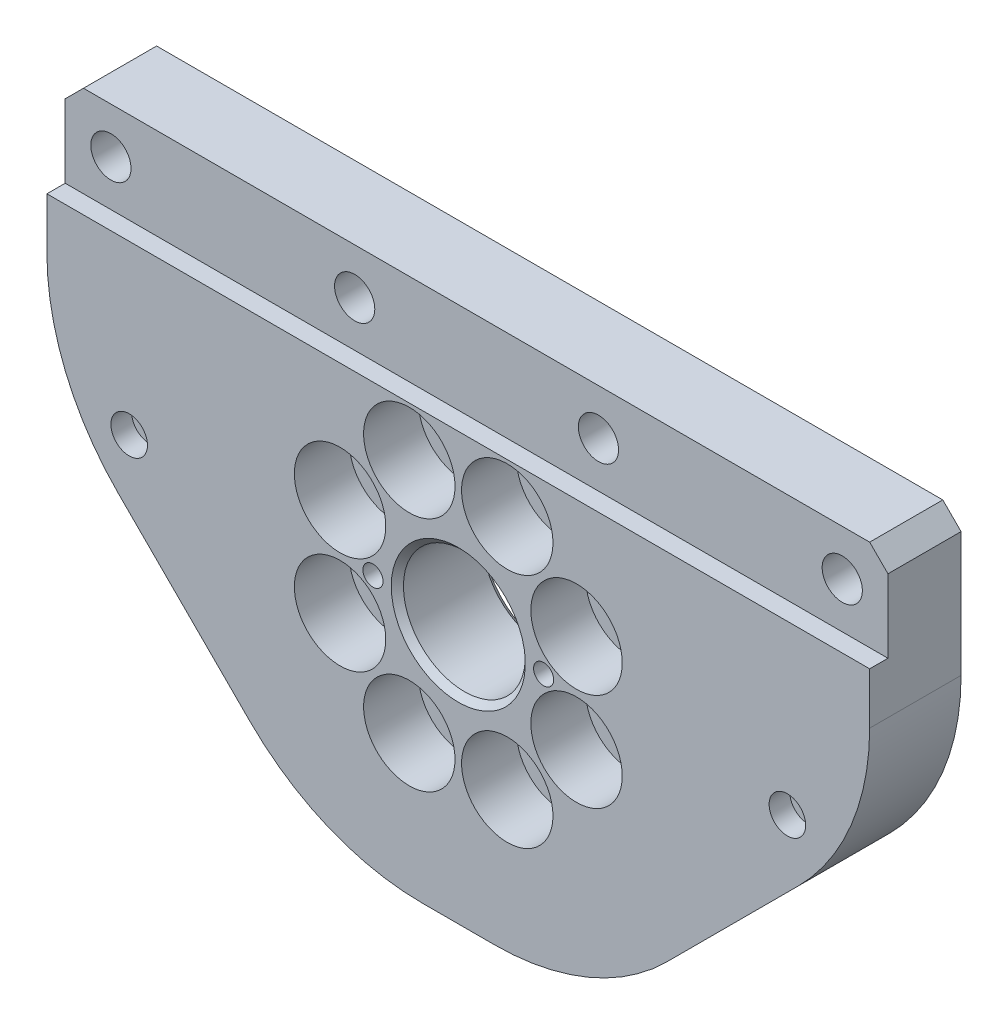
from build123d import *

# Parameters (mm, degrees)
SKETCH_1_R                  = 10
EXTRUDE_1_DEPTH             = 7.5
HOLE_WIZARD_2_D             = 9
HOLE_WIZARD_2_CBORE_D       = 15
HOLE_WIZARD_2_CBORE_DEPTH   = 9
CHAMFER_1_SIZE              = 1
PATTERN_CIRCULAR_1_COUNT    = 8
HOLE_WIZARD_2_2_D           = 3.4
HOLE_WIZARD_2_2_CBORE_D     = 6
HOLE_WIZARD_2_2_CBORE_DEPTH = 3.4
HOLE_WIZARD_8_0_8_1_D       = 8
HOLE_WIZARD_8_0_8_1_DEPTH   = 8
HOLE_WIZARD_8_0_8_1_TIP     = 2.403442476
HOLE_WIZARD_M4_1_D          = 3.3
SKETCH_10_W                 = 135
SKETCH_10_H                 = 15
CUT_EXTRUDE_1_DEPTH         = 3
HOLE_WIZARD_3_D             = 6.6
HOLE_WIZARD_3_CBORE_D       = 11
HOLE_WIZARD_3_CBORE_DEPTH   = 6.8
CHAMFER_2_SIZE              = 3


with BuildPart() as part:
    # 草图1 → 凸台-拉伸1 (new, symmetric)
    with BuildSketch(Plane.XY):
        with BuildLine():
            Line((-55.784271247, -9.215728753), (-34.215728753, -30.784271247))
            ThreePointArc((-34.215728753, -30.784271247), (-21.2387948, -39.4551813), (-5.931457505, -42.5))
            Line((-5.931457505, -42.5), (5.931457505, -42.5))
            ThreePointArc((5.931457505, -42.5), (21.2387948, -39.4551813), (34.215728753, -30.784271247))
            Line((34.215728753, -30.784271247), (55.784271247, -9.215728753))
            ThreePointArc((55.784271247, -9.215728753), (64.4551813, 3.7612052), (67.5, 19.068542495))
            Line((67.5, 19.068542495), (67.5, 42.5))
            Line((67.5, 42.5), (-67.5, 42.5))
            Line((-67.5, 42.5), (-67.5, 19.068542495))
            ThreePointArc((-67.5, 19.068542495), (-64.4551813, 3.7612052), (-55.784271247, -9.215728753))
        make_face()
        Circle(SKETCH_1_R, mode=Mode.SUBTRACT)
    extrude(amount=EXTRUDE_1_DEPTH, both=True)

    # Hole Wizard 2 (through all)
    with Locations(Plane.XY.offset(7.5)):
        with Locations((-8.03635208, 19.401470183)):
            hole_wizard_2 = CounterBoreHole(HOLE_WIZARD_2_D / 2, HOLE_WIZARD_2_CBORE_D / 2, HOLE_WIZARD_2_CBORE_DEPTH)

    # 倒角1
    chamfer_1_edges = [part.edges().sort_by_distance(p)[0] for p in [
        (-10, 0, -7.5),
        (-10, 0, 7.5),
    ]]
    chamfer(chamfer_1_edges, length=CHAMFER_1_SIZE)

    # 阵列(圆周)1: Hole Wizard 2 ×8 about axis
    pattern_circular_1_axis = Axis((0, 0, 0), (0, 0, 1))
    for i in range(1, PATTERN_CIRCULAR_1_COUNT):
        add(hole_wizard_2.rotate(pattern_circular_1_axis, i * 360 / PATTERN_CIRCULAR_1_COUNT), mode=Mode.SUBTRACT)

    # Hole Wizard 2 2 (through all)
    with Locations(Plane.XY.offset(7.5)):
        with Locations((-54, 0), (54, 0)):
            CounterBoreHole(HOLE_WIZARD_2_2_D / 2, HOLE_WIZARD_2_2_CBORE_D / 2, HOLE_WIZARD_2_2_CBORE_DEPTH)

    # Ø8.0 (8) 直径孔1
    with Locations(Plane(origin=(0, 0, -7.5), x_dir=(-1, 0, 0), z_dir=(0, 0, -1))):
        with Locations((-54, 0), (54, 0)):
            Hole(HOLE_WIZARD_8_0_8_1_D / 2, depth=HOLE_WIZARD_8_0_8_1_DEPTH)
            with Locations((0, 0, -(HOLE_WIZARD_8_0_8_1_DEPTH + HOLE_WIZARD_8_0_8_1_TIP / 2))):  # 118° drill point
                Cone(0, HOLE_WIZARD_8_0_8_1_D / 2, HOLE_WIZARD_8_0_8_1_TIP, mode=Mode.SUBTRACT)

    # M4 螺纹孔1 (through all)
    with Locations(Plane(origin=(0, 0, -7.5), x_dir=(-1, 0, 0), z_dir=(0, 0, -1))):
        with Locations((-14, 0), (14, 0)):
            Hole(HOLE_WIZARD_M4_1_D / 2)

    # 草图10 → 切除-拉伸1 (cut)
    with BuildSketch(Plane.XY.offset(7.5)):
        with Locations((0, 35)):
            Rectangle(SKETCH_10_W, SKETCH_10_H)
    extrude(amount=-CUT_EXTRUDE_1_DEPTH, mode=Mode.SUBTRACT)

    # 打孔尺寸(%根据)内六角圆柱头螺钉的类型3 (through all)
    with Locations(Plane(origin=(0, 0, -7.5), x_dir=(-1, 0, 0), z_dir=(0, 0, -1))):
        with Locations((-20, 35), (-60, 35), (60, 35), (20, 35)):
            CounterBoreHole(HOLE_WIZARD_3_D / 2, HOLE_WIZARD_3_CBORE_D / 2, HOLE_WIZARD_3_CBORE_DEPTH)

    # 倒角2
    chamfer_2_edges = [part.edges().sort_by_distance(p)[0] for p in [
        (-67.5, 42.5, -1.5),
        (67.5, 42.5, -1.5),
    ]]
    chamfer(chamfer_2_edges, length=CHAMFER_2_SIZE)


solid = part.part
